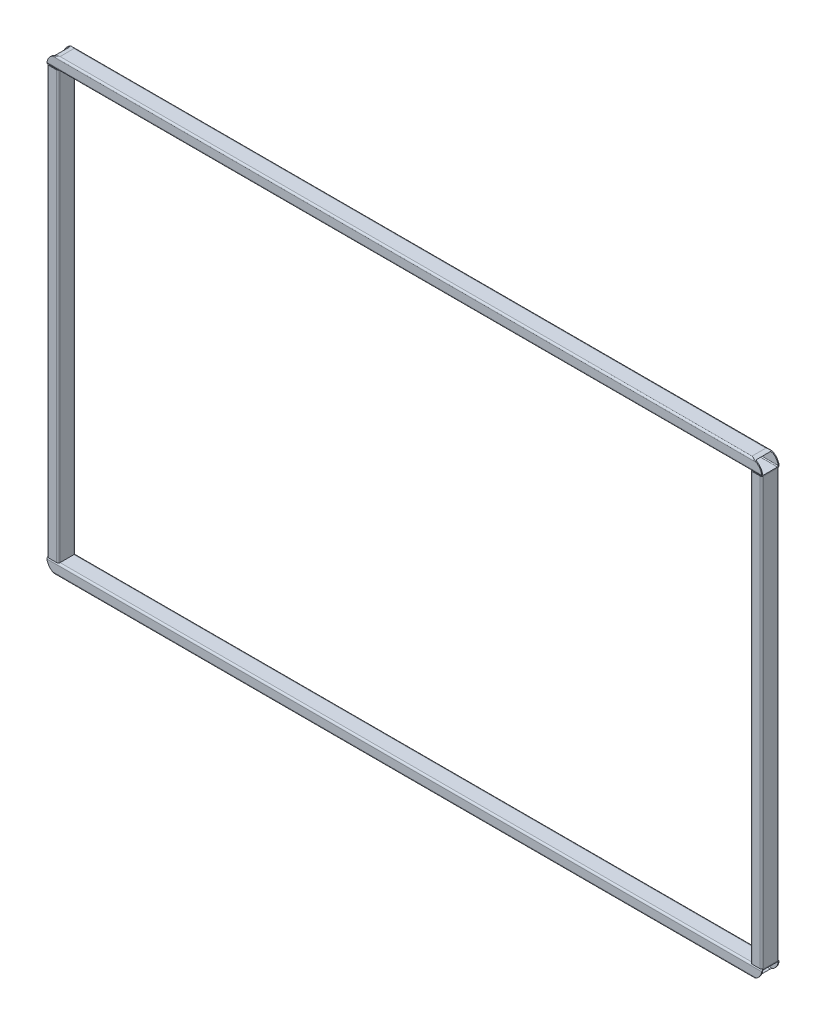
from build123d import *

# Parameters (mm, degrees)
GB_6728_1986_RECT_HOLLOW_SECTION_060_X_4_DEPTH      = 2460
GB_6728_1986_RECT_HOLLOW_SECTION_060_X_4_DEPTH_BACK = 20
GB_6728_1986_RECT_HOLLOW_SECTION_060_2_DEPTH        = 2480
GB_6728_1986_RECT_HOLLOW_SECTION_060_3_DEPTH        = 1522
GB_6728_1986_RECT_HOLLOW_SECTION_060_5_DEPTH        = 1522
CUT_EXTRUDE1_DEPTH                                  = 2877.6821166058676


with BuildPart() as part:
    # Sketch14 → GB/6728-1986 rect hollow section 060 X 40 X 3(1) (new, two sides: drawn at the far end of the back side and taken through both)
    with BuildSketch(Plane(origin=(0, 1520, 0), x_dir=(0, 1, 3.49e-15), z_dir=(1, 0, 0)).offset(-GB_6728_1986_RECT_HOLLOW_SECTION_060_X_4_DEPTH_BACK)):
        with BuildLine():
            Line((-14, -30), (14, -30))
            ThreePointArc((14, -30), (18.242640687119284, -28.242640687119284), (20.000000000000004, -24))
            Line((20.000000000000004, -24), (20.000000000000004, 24))
            ThreePointArc((20.000000000000004, 24), (18.242640687119287, 28.242640687119287), (14, 30))
            Line((14, 30), (-14, 30))
            ThreePointArc((-14, 30), (-18.242640687119284, 28.242640687119284), (-20.000000000000004, 24))
            Line((-20.000000000000004, 24), (-20.000000000000004, -24))
            ThreePointArc((-20.000000000000004, -24), (-18.242640687119287, -28.242640687119287), (-14, -30))
        make_face()
        with BuildLine():
            Line((-14, -27.000000000000004), (14, -27.000000000000004))
            ThreePointArc((14, -27.000000000000004), (16.121320343559645, -26.121320343559645), (17, -24))
            Line((17, -24), (17, 24))
            ThreePointArc((17, 24), (16.121320343559642, 26.121320343559642), (14, 27.000000000000004))
            Line((14, 27.000000000000004), (-14, 27.000000000000004))
            ThreePointArc((-14, 27.000000000000004), (-16.121320343559645, 26.121320343559645), (-17, 24))
            Line((-17, 24), (-17, -24))
            ThreePointArc((-17, -24), (-16.121320343559642, -26.121320343559642), (-14, -27.000000000000004))
        make_face(mode=Mode.SUBTRACT)
    extrude(amount=GB_6728_1986_RECT_HOLLOW_SECTION_060_X_4_DEPTH + GB_6728_1986_RECT_HOLLOW_SECTION_060_X_4_DEPTH_BACK)


with BuildPart() as body_2:
    # Sketch14 on segment 2 (carried to segment 2) → GB_6728-1986 rect hollow section 060 2 (new body)
    with BuildSketch(Plane.YZ.offset(-20)):
        with BuildLine():
            Line((-14, -30), (14, -30))
            ThreePointArc((14, -30), (18.242640687119284, -28.242640687119284), (20.000000000000004, -24))
            Line((20.000000000000004, -24), (20.000000000000004, 24))
            ThreePointArc((20.000000000000004, 24), (18.242640687119287, 28.242640687119287), (14, 30))
            Line((14, 30), (-14, 30))
            ThreePointArc((-14, 30), (-18.242640687119284, 28.242640687119284), (-20.000000000000004, 24))
            Line((-20.000000000000004, 24), (-20.000000000000004, -24))
            ThreePointArc((-20.000000000000004, -24), (-18.242640687119287, -28.242640687119287), (-14, -30))
        make_face()
        with BuildLine():
            Line((-14, -27.000000000000004), (14, -27.000000000000004))
            ThreePointArc((14, -27.000000000000004), (16.121320343559645, -26.121320343559645), (17, -24))
            Line((17, -24), (17, 24))
            ThreePointArc((17, 24), (16.121320343559642, 26.121320343559642), (14, 27.000000000000004))
            Line((14, 27.000000000000004), (-14, 27.000000000000004))
            ThreePointArc((-14, 27.000000000000004), (-16.121320343559645, 26.121320343559645), (-17, 24))
            Line((-17, 24), (-17, -24))
            ThreePointArc((-17, -24), (-16.121320343559642, -26.121320343559642), (-14, -27.000000000000004))
        make_face(mode=Mode.SUBTRACT)
    extrude(amount=GB_6728_1986_RECT_HOLLOW_SECTION_060_2_DEPTH)


with BuildPart() as body_3:
    # Sketch14 on segment 3 (carried to segment 3) → GB_6728-1986 rect hollow section 060 3 (new body)
    with BuildSketch(Plane(origin=(0, -1, 0), x_dir=(-1, 0, 0), z_dir=(0, 1, 0))):
        with BuildLine():
            Line((-14, -30), (14, -30))
            ThreePointArc((14, -30), (18.242640687119284, -28.242640687119284), (20.000000000000004, -24))
            Line((20.000000000000004, -24), (20.000000000000004, 24))
            ThreePointArc((20.000000000000004, 24), (18.242640687119287, 28.242640687119287), (14, 30))
            Line((14, 30), (-14, 30))
            ThreePointArc((-14, 30), (-18.242640687119284, 28.242640687119284), (-20.000000000000004, 24))
            Line((-20.000000000000004, 24), (-20.000000000000004, -24))
            ThreePointArc((-20.000000000000004, -24), (-18.242640687119287, -28.242640687119287), (-14, -30))
        make_face()
        with BuildLine():
            Line((-14, -27.000000000000004), (14, -27.000000000000004))
            ThreePointArc((14, -27.000000000000004), (16.121320343559645, -26.121320343559645), (17, -24))
            Line((17, -24), (17, 24))
            ThreePointArc((17, 24), (16.121320343559642, 26.121320343559642), (14, 27.000000000000004))
            Line((14, 27.000000000000004), (-14, 27.000000000000004))
            ThreePointArc((-14, 27.000000000000004), (-16.121320343559645, 26.121320343559645), (-17, 24))
            Line((-17, 24), (-17, -24))
            ThreePointArc((-17, -24), (-16.121320343559642, -26.121320343559642), (-14, -27.000000000000004))
        make_face(mode=Mode.SUBTRACT)
    extrude(amount=GB_6728_1986_RECT_HOLLOW_SECTION_060_3_DEPTH)

    # GB_6728-1986 rect hollow section 060 3 e
    split(bisect_by=Plane(origin=(0, 20, 0), x_dir=(-1, 0, 0), z_dir=(0, 1, 0)), keep=Keep.TOP)

    # GB_6728-1986 rect hollow section 060 4
    split(bisect_by=Plane.XZ.offset(-1500), keep=Keep.TOP)


with BuildPart() as body_4:
    # Sketch14 on segment 4 (carried to segment 4) → GB_6728-1986 rect hollow section 060 5 (new body)
    with BuildSketch(Plane(origin=(2440, -1, 0), x_dir=(-1, 0, 0), z_dir=(0, 1, 0))):
        with BuildLine():
            Line((-14, -30), (14, -30))
            ThreePointArc((14, -30), (18.242640687119284, -28.242640687119284), (20.000000000000004, -24))
            Line((20.000000000000004, -24), (20.000000000000004, 24))
            ThreePointArc((20.000000000000004, 24), (18.242640687119287, 28.242640687119287), (14, 30))
            Line((14, 30), (-14, 30))
            ThreePointArc((-14, 30), (-18.242640687119284, 28.242640687119284), (-20.000000000000004, 24))
            Line((-20.000000000000004, 24), (-20.000000000000004, -24))
            ThreePointArc((-20.000000000000004, -24), (-18.242640687119287, -28.242640687119287), (-14, -30))
        make_face()
        with BuildLine():
            Line((-14, -27.000000000000004), (14, -27.000000000000004))
            ThreePointArc((14, -27.000000000000004), (16.121320343559645, -26.121320343559645), (17, -24))
            Line((17, -24), (17, 24))
            ThreePointArc((17, 24), (16.121320343559642, 26.121320343559642), (14, 27.000000000000004))
            Line((14, 27.000000000000004), (-14, 27.000000000000004))
            ThreePointArc((-14, 27.000000000000004), (-16.121320343559645, 26.121320343559645), (-17, 24))
            Line((-17, 24), (-17, -24))
            ThreePointArc((-17, -24), (-16.121320343559642, -26.121320343559642), (-14, -27.000000000000004))
        make_face(mode=Mode.SUBTRACT)
    extrude(amount=GB_6728_1986_RECT_HOLLOW_SECTION_060_5_DEPTH)

    # GB_6728-1986 rect hollow section 060 5 e
    split(bisect_by=Plane(origin=(2440, 20, 0), x_dir=(-1, 0, 0), z_dir=(0, 1, 0)), keep=Keep.TOP)

    # GB_6728-1986 rect hollow section 060 6
    split(bisect_by=Plane(origin=(2440, 1500, 0), x_dir=(1, 0, 0), z_dir=(0, -1, 0)), keep=Keep.TOP)


with BuildPart() as cut_extrude1_tool:
    # Sketch2 → Cut-Extrude1 (new, through all)
    with BuildSketch(Plane(origin=(0, 1470.0000000000052, 29.999999999994724), x_dir=(1, 0, 0), z_dir=(0, 0, 1))):
        with BuildLine():
            Line((-20.000000000000014, -1450.0000000000052), (-20.000000000000018, -1490.0000000000052))
            Line((-20.000000000000018, -1490.0000000000052), (20.000000000000018, -1490.0000000000052))
            ThreePointArc((20.000000000000018, -1490.0000000000052), (-8.284271247461913, -1478.2842712474671), (-20.000000000000014, -1450.0000000000052))
        make_face()
        with BuildLine():
            Line((-20.000000000000018, 69.99999999999473), (20.000000000000018, 69.99999999999473))
            ThreePointArc((20.000000000000018, 69.99999999999473), (-8.284271247461902, 58.284271247456616), (-20.000000000000014, 29.9999999999947))
            Line((-20.000000000000014, 29.9999999999947), (-20.000000000000018, 69.99999999999473))
        make_face()
        with BuildLine():
            Line((2460, -1490.0000000000052), (2420, -1490.0000000000052))
            ThreePointArc((2420, -1490.0000000000052), (2448.284271247462, -1478.2842712474671), (2460, -1450.0000000000052))
            Line((2460, -1450.0000000000052), (2460, -1490.0000000000052))
        make_face()
        with BuildLine():
            Line((2460, 29.9999999999947), (2460, 69.99999999999473))
            Line((2460, 69.99999999999473), (2420, 69.99999999999473))
            ThreePointArc((2420, 69.99999999999473), (2448.284271247462, 58.2842712474566), (2460, 29.9999999999947))
        make_face()
    extrude(amount=-CUT_EXTRUDE1_DEPTH)


with BuildPart() as part_1:
    add(part.part)

    # Cut-Extrude1: cut by cut_extrude1_tool
    add(cut_extrude1_tool.part, mode=Mode.SUBTRACT)


with BuildPart() as body_2_1:
    add(body_2.part)

    # Cut-Extrude1: cut by cut_extrude1_tool
    add(cut_extrude1_tool.part, mode=Mode.SUBTRACT)


solid = Compound([body_3.part, body_4.part, part_1.part, body_2_1.part])
